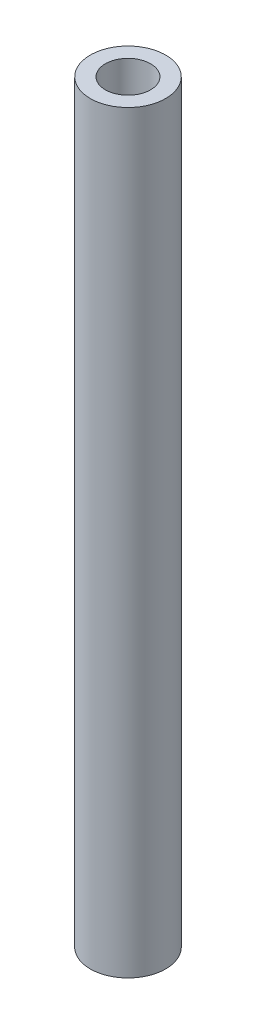
from build123d import *

# Parameters (mm, degrees)
SKETCH_1_R      = 5
SKETCH_1_R_2    = 3
EXTRUDE_1_DEPTH = 100


with BuildPart() as part:
    # 草图1 → 凸台-拉伸1 (new body)
    with BuildSketch(Plane(origin=(0, 0, 0), x_dir=(1, 0, 0), z_dir=(0, 1, 0))):
        with Locations(Location((0, 0, 0), (0, 0, 270))):
            Circle(SKETCH_1_R)
        with Locations(Location((0, 0, 0), (0, 0, 270))):
            Circle(SKETCH_1_R_2, mode=Mode.SUBTRACT)
    extrude(amount=EXTRUDE_1_DEPTH)


solid = part.part
